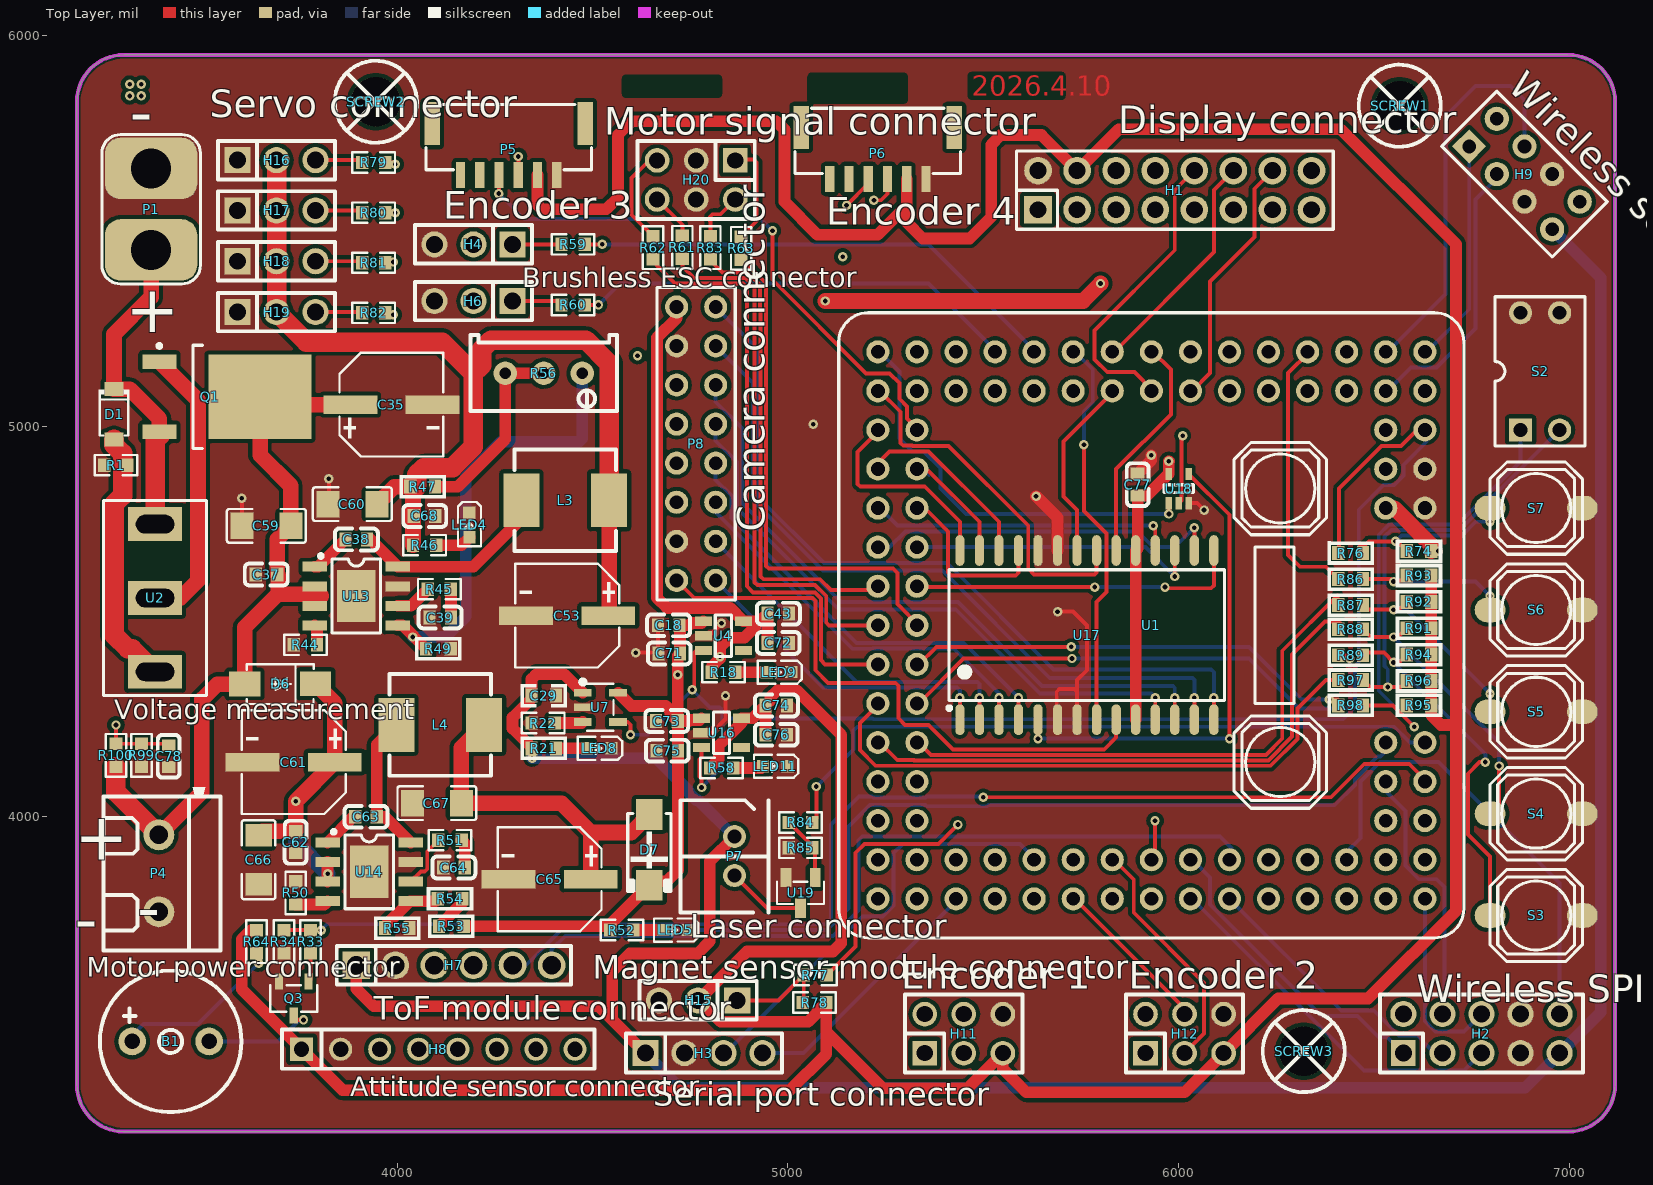
[diagram p0: Top Layer view]
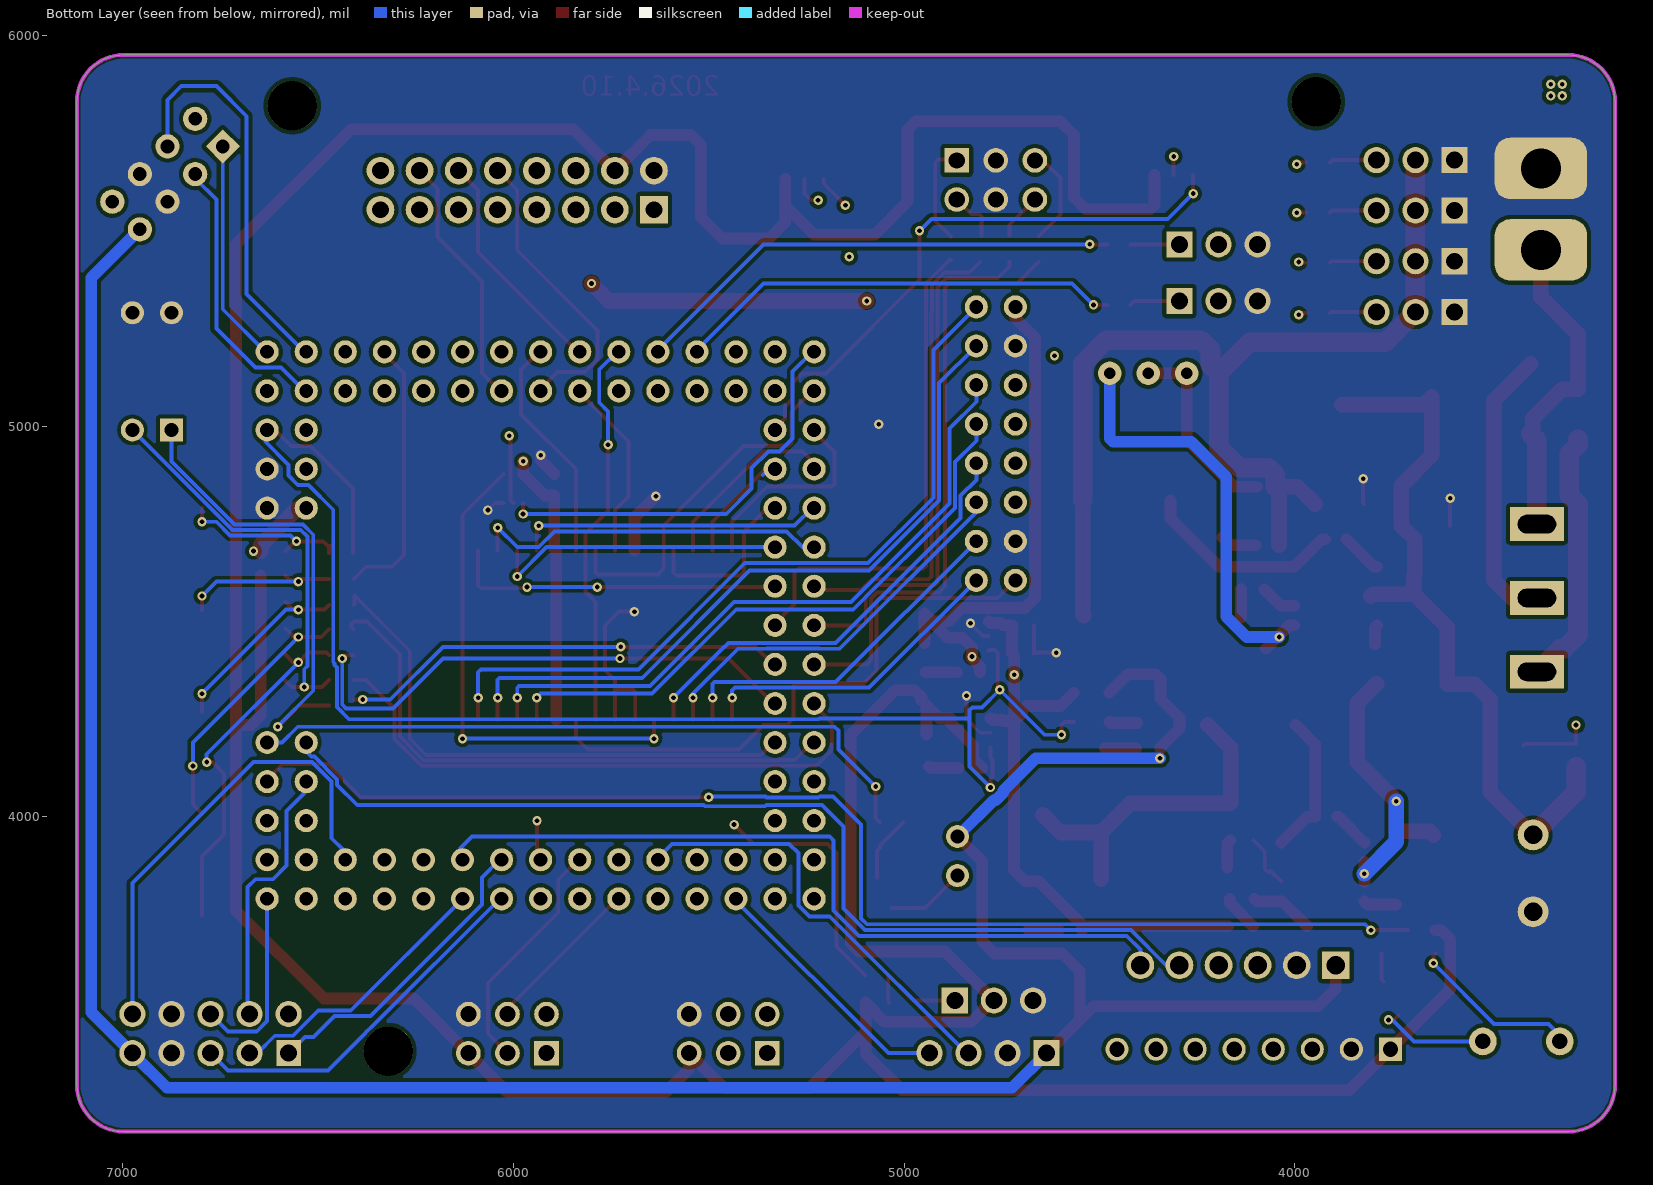
[diagram p1: Bottom Layer view, seen from below]
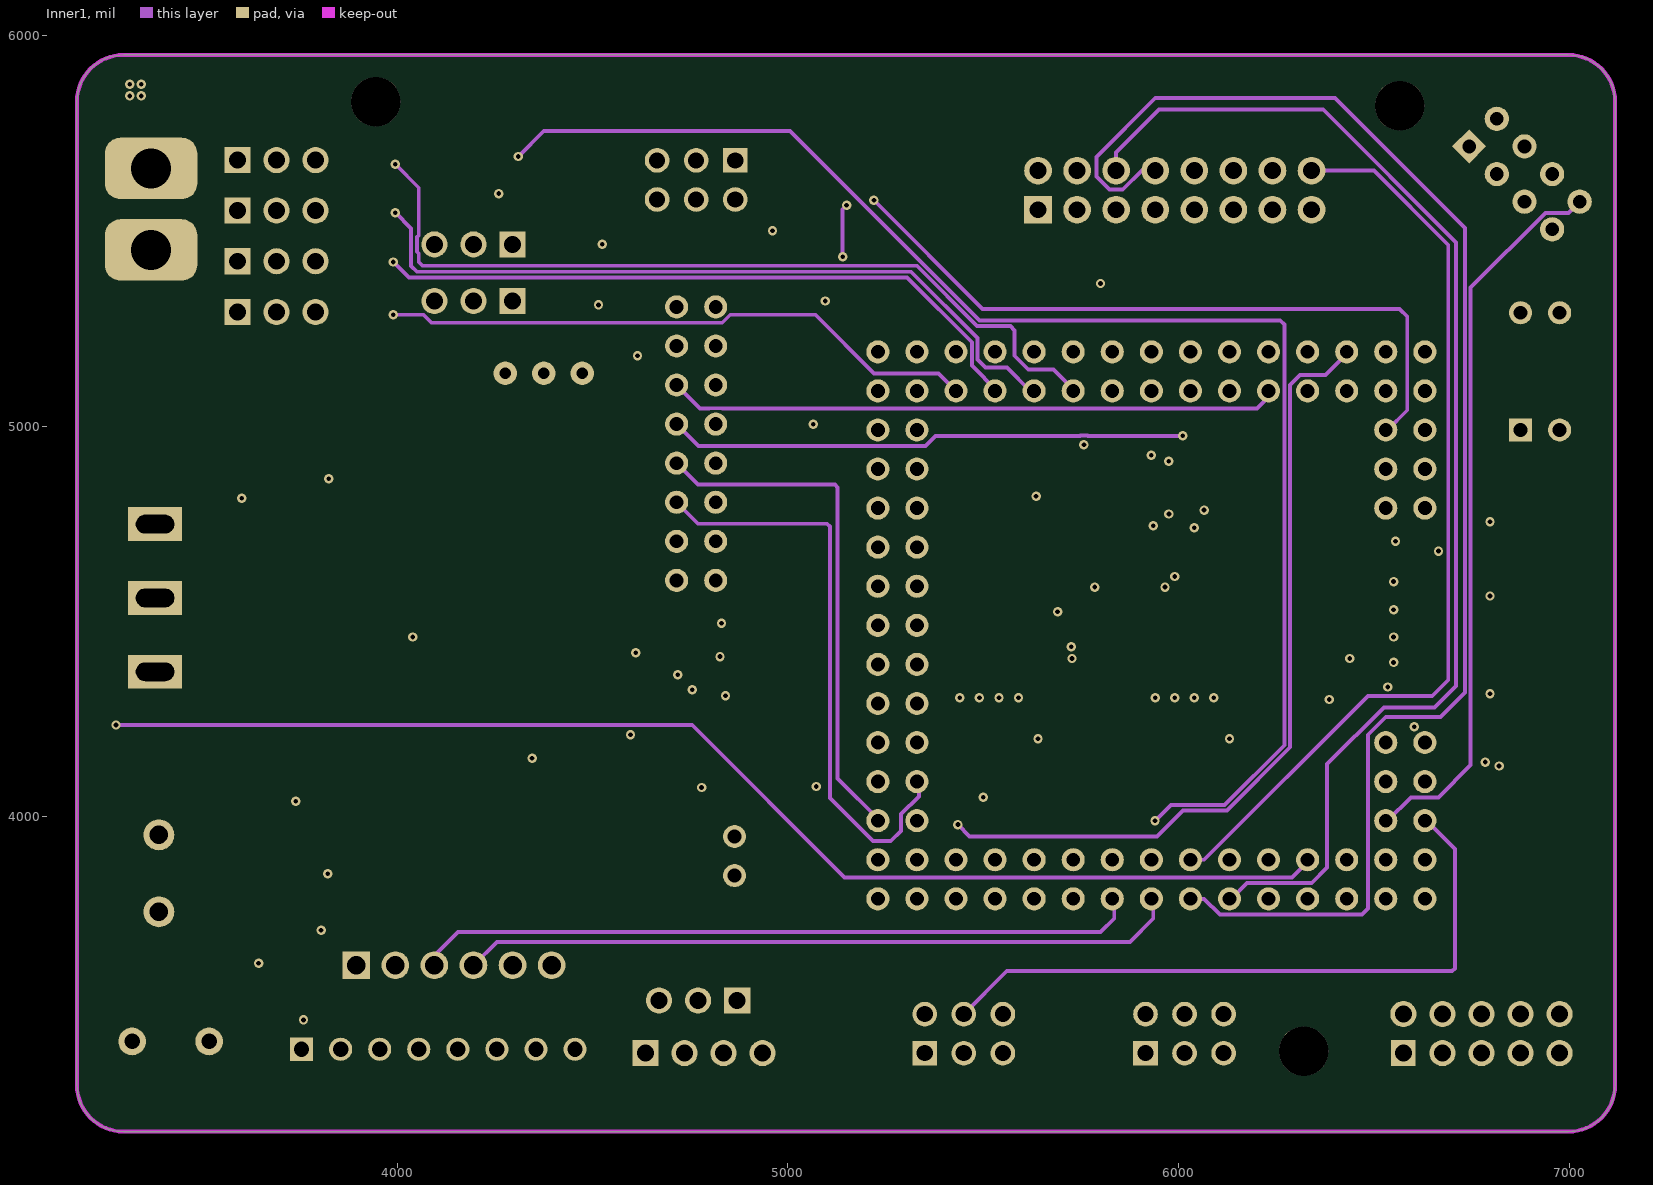
[diagram p2: Inner1]
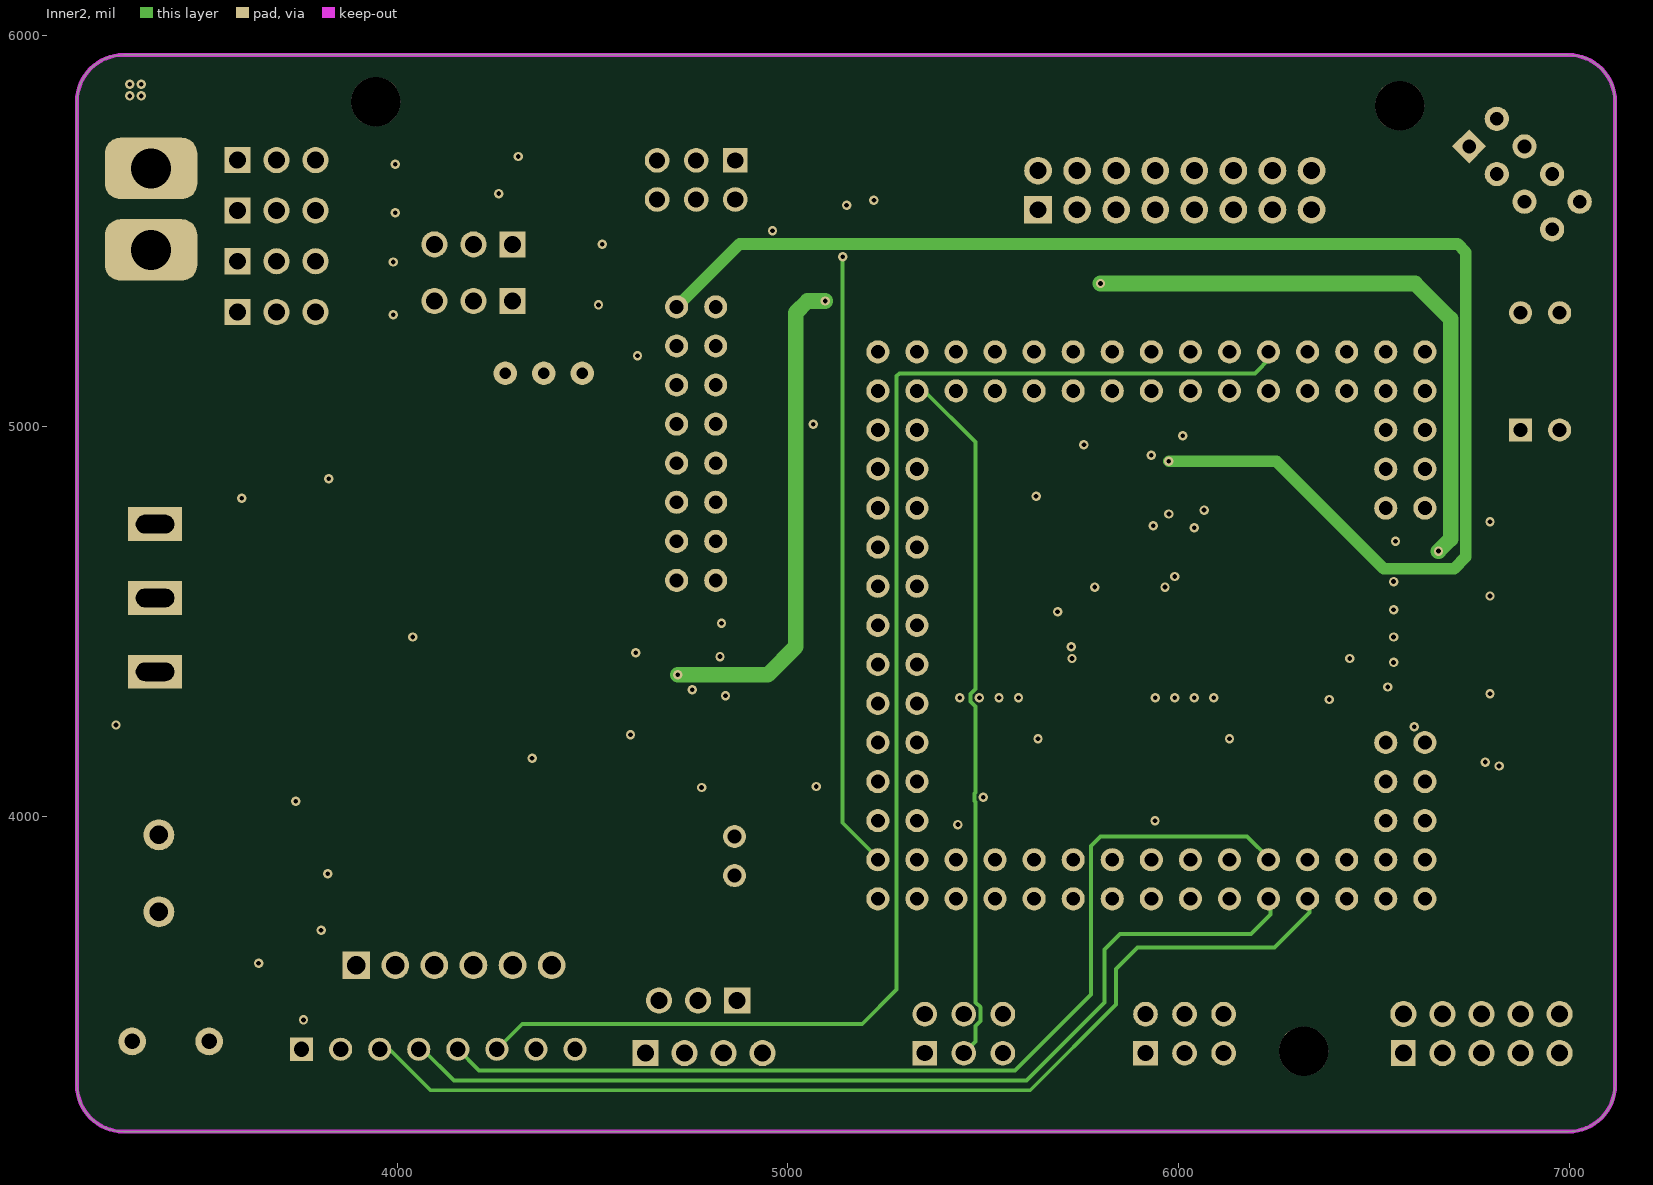
[diagram p3: Inner2]
# Altium PCB MISC49918.pcbdoc (part 1 of 2)
Units mil, origin at the board's own origin, x right, y up, seen from the top; angles counter-clockwise.
Board outline 3937.01 x 2755.91 mil, 4 copper layers (Top Layer, Inner1, Inner2, Bottom Layer), stack 62.447 mil thick; 130 components, 134 nets, 493 pads, 82 vias.

## Layer stack, top to bottom
Top Layer: signal copper 1.378
Dielectric1: surface 8.283, 7628 RC49% 8.6mil, Dk 0
Inner1: signal copper 0.598
Dielectric2: surface 41.929, 1.1mm H/HOZ Copper, Dk 0
Inner2: signal copper 0.598
Dielectric3: surface 8.283, 7628 RC49% 8.6mil, Dk 0
Bottom Layer: signal copper 1.378

## Board outline
3300,5950 ccw(c3300,5830) 3180,5830 3180,3314.09 ccw(c3300,3314.09) 3300,3194.09 6997.01,3194.09 ccw(c6997.01,3314.09) 7117.01,3314.09 7117.01,5830 ccw(c6997.01,5830) 6997.01,5950

## Design rules (kind name [scope] priority, off if disabled: settings)
BoardOutlineClearance copperThickness2oz_1 [All] p2 off: genericclearance=7.99 ignorepadtopadclearanceinfootprint=FALSE except(0: Arc-SplitContinuation Track-SplitContinuation SMDPad-SplitContinuation THPad-SplitContinuation Via-SplitContinuation Fill-SplitContinuation Region-SplitContinuation Poly-SplitContinuation Text-SplitContinuation Hole-SplitContinuation; 5.98: Arc-CutoutEdge SMDPad-CutoutEdge THPad-CutoutEdge Via-CutoutEdge Fill-CutoutEdge Region-CutoutEdge Text-CutoutEdge; 6.93: Hole-OutlineEdge Hole-CutoutEdge; 10: Poly-OutlineEdge Poly-CutoutEdge; 11.81: Arc-OutlineEdge Track-OutlineEdge SMDPad-OutlineEdge THPad-OutlineEdge Via-OutlineEdge Fill-OutlineEdge Region-OutlineEdge Text-OutlineEdge Track-CutoutEdge)
BoardOutlineClearance Plane_innerPlane_1 [All] p4 off: genericclearance=4.02 ignorepadtopadclearanceinfootprint=FALSE except(0: Arc-SplitContinuation Track-SplitContinuation SMDPad-SplitContinuation THPad-SplitContinuation Via-SplitContinuation Fill-SplitContinuation Region-SplitContinuation Poly-SplitContinuation Text-SplitContinuation Hole-SplitContinuation; 6: SMDPad-CutoutEdge THPad-CutoutEdge Via-CutoutEdge Fill-CutoutEdge Region-CutoutEdge Text-CutoutEdge; 6.93: Hole-OutlineEdge Hole-CutoutEdge; 10: Poly-OutlineEdge Poly-CutoutEdge; 11.8: Arc-OutlineEdge Track-OutlineEdge SMDPad-OutlineEdge THPad-OutlineEdge Via-OutlineEdge Fill-OutlineEdge Region-OutlineEdge Text-OutlineEdge; 11.81: Arc-CutoutEdge Track-CutoutEdge)
BoardOutlineClearance Copper_copperRegion_1 [All] p6 off: genericclearance=4.02 ignorepadtopadclearanceinfootprint=FALSE except(0: Arc-SplitContinuation Track-SplitContinuation SMDPad-SplitContinuation THPad-SplitContinuation Via-SplitContinuation Fill-SplitContinuation Region-SplitContinuation Poly-SplitContinuation Text-SplitContinuation Hole-SplitContinuation; 6: SMDPad-CutoutEdge THPad-CutoutEdge Via-CutoutEdge Fill-CutoutEdge Region-CutoutEdge Text-CutoutEdge; 6.93: Hole-OutlineEdge Hole-CutoutEdge; 10: Poly-OutlineEdge Poly-CutoutEdge; 11.8: Arc-OutlineEdge Track-OutlineEdge SMDPad-OutlineEdge THPad-OutlineEdge Via-OutlineEdge Fill-OutlineEdge Region-OutlineEdge Text-OutlineEdge; 11.81: Arc-CutoutEdge Track-CutoutEdge)
BoardOutlineClearance copperThickness1oz_1 [All] p8: genericclearance=4.02 ignorepadtopadclearanceinfootprint=FALSE except(0: Arc-SplitContinuation Track-SplitContinuation SMDPad-SplitContinuation THPad-SplitContinuation Via-SplitContinuation Fill-SplitContinuation Region-SplitContinuation Poly-SplitContinuation Text-SplitContinuation Hole-SplitContinuation; 6: SMDPad-CutoutEdge THPad-CutoutEdge Via-CutoutEdge Fill-CutoutEdge Region-CutoutEdge Text-CutoutEdge; 6.93: Hole-OutlineEdge Hole-CutoutEdge; 10: Poly-OutlineEdge Poly-CutoutEdge; 11.8: Arc-OutlineEdge Track-OutlineEdge SMDPad-OutlineEdge THPad-OutlineEdge Via-OutlineEdge Fill-OutlineEdge Region-OutlineEdge Text-OutlineEdge; 11.81: Arc-CutoutEdge Track-CutoutEdge)
Clearance copperThickness2oz [All] p1 off: gap=7.99 ignorepadtopadclearanceinfootprint=FALSE except(5.98: SMDPad-Track SMDPad-SMDPad THPad-Track SMDPad-THPad THPad-THPad Track-Via SMDPad-Via THPad-Via Via-Via Fill-Track Region-Track Fill-SMDPad Region-SMDPad Fill-THPad Region-THPad Fill-Via Region-Via Fill-Fill Fill-Region Region-Region Arc-Track Arc-SMDPad Arc-THPad Arc-Via Fill-Arc Region-Arc Arc-Arc Text-Track SMDPad-Text Text-THPad Text-Via Fill-Text Region-Text Arc-Text Text-Text; 6.93: Hole-Track Hole-SMDPad Hole-THPad Hole-Via Fill-Hole Region-Hole Hole-Arc Hole-Text; 10: Poly-Track Poly-SMDPad Poly-THPad Poly-Via Poly-Fill Poly-Region Poly-Poly Poly-Arc Poly-Text Poly-Hole)
Clearance Plane_innerPlane [All] p3 off: gap=4.02 ignorepadtopadclearanceinfootprint=FALSE except(5.98: SMDPad-Track SMDPad-SMDPad THPad-Track SMDPad-THPad THPad-THPad Track-Via SMDPad-Via THPad-Via Via-Via Fill-Track Region-Track Fill-SMDPad Region-SMDPad Fill-THPad Region-THPad Fill-Via Region-Via Fill-Fill Fill-Region Region-Region; 6: Arc-Track Arc-SMDPad Arc-THPad Arc-Via Fill-Arc Region-Arc Arc-Arc Text-Track SMDPad-Text Text-THPad Text-Via Fill-Text Region-Text Arc-Text Text-Text; 6.93: Hole-Track Hole-SMDPad Hole-THPad Hole-Via Fill-Hole Region-Hole Hole-Arc Hole-Text; 10: Poly-Track Poly-SMDPad Poly-THPad Poly-Via Poly-Fill Poly-Region Poly-Poly Poly-Arc Poly-Text Poly-Hole)
Clearance Copper_copperRegion [All] p5 off: gap=4.02 ignorepadtopadclearanceinfootprint=FALSE except(5.98: SMDPad-Track SMDPad-SMDPad THPad-Track SMDPad-THPad THPad-THPad Track-Via SMDPad-Via THPad-Via Via-Via Fill-Track Region-Track Fill-SMDPad Region-SMDPad Fill-THPad Region-THPad Fill-Via Region-Via Fill-Fill Fill-Region Region-Region; 6: Arc-Track Arc-SMDPad Arc-THPad Arc-Via Fill-Arc Region-Arc Arc-Arc Text-Track SMDPad-Text Text-THPad Text-Via Fill-Text Region-Text Arc-Text Text-Text; 6.93: Hole-Track Hole-SMDPad Hole-THPad Hole-Via Fill-Hole Region-Hole Hole-Arc Hole-Text; 10: Poly-Track Poly-SMDPad Poly-THPad Poly-Via Poly-Fill Poly-Region Poly-Poly Poly-Arc Poly-Text Poly-Hole)
Clearance copperThickness1oz [All] p7: gap=4.02 ignorepadtopadclearanceinfootprint=FALSE except(5.98: SMDPad-Track SMDPad-SMDPad THPad-Track SMDPad-THPad THPad-THPad Track-Via SMDPad-Via THPad-Via Via-Via Fill-Track Region-Track Fill-SMDPad Region-SMDPad Fill-THPad Region-THPad Fill-Via Region-Via Fill-Fill Fill-Region Region-Region; 6: Arc-Track Arc-SMDPad Arc-THPad Arc-Via Fill-Arc Region-Arc Arc-Arc Text-Track SMDPad-Text Text-THPad Text-Via Fill-Text Region-Text Arc-Text Text-Text; 6.93: Hole-Track Hole-SMDPad Hole-THPad Hole-Via Fill-Hole Region-Hole Hole-Arc Hole-Text; 10: Poly-Track Poly-SMDPad Poly-THPad Poly-Via Poly-Fill Poly-Region Poly-Poly Poly-Arc Poly-Text Poly-Hole)
DiffPairsRouting differentialPair [All] p1: maxlimit=6 minlimit=6 mostfreqgap=6 toplayer_minwidth=5 toplayer_prefwidth=10 toplayer_maxwidth=100 toplayer_mingap=6 toplayer_prefgap=6 toplayer_maxgap=6 midlayer1_minwidth=5 midlayer1_prefwidth=10 midlayer1_maxwidth=100 midlayer1_mingap=6 midlayer1_prefgap=6 midlayer1_maxgap=6 midlayer2_minwidth=5 midlayer2_prefwidth=10 midlayer2_maxwidth=100 midlayer2_mingap=6 midlayer2_prefgap=6 midlayer2_maxgap=6 bottomlayer_minwidth=5 bottomlayer_prefwidth=10 bottomlayer_maxwidth=100 bottomlayer_mingap=6 bottomlayer_prefgap=6 bottomlayer_maxgap=6 maxuncoupledlength=10
HoleToHoleClearance otherClearance [All] p1: gap=11.81 allowstackedmicrovias=TRUE
Length netLength [All] p1: minlimit=0 maxlimit=0
PasteMaskExpansion pasteMaskExpansion [All] p1: expansion=0
PlaneConnect innerPlane [All] p1: planeconnectstyle=Relief reliefexpansion=20 reliefentries=4 reliefconductorwidth=10 reliefairgap=10
PolygonConnect copperRegion [All] p1: connectstyle=Direct reliefconductorwidth=10 reliefentries=4 polygonreliefangle="90 Angle" airgapwidth=10 via.connectstyle=Relief via.reliefconductorwidth=10 via.reliefentries=4 via.polygonreliefangle="90 Angle" via.airgapwidth=10
RoutingVias viaSize [All] p1: holewidth=12.01 width=24.02 viastyle="Through Hole" minholewidth=11.81 minwidth=19.68 maxholewidth=248.03 maxwidth=393.7
SolderMaskExpansion solderMaskExpansion [IsVia] p1: expansion=-1000 istentingtop=TRUE
SolderMaskExpansion solderMaskExpansion [All] p2: expansion=2 istentingtop=FALSE
Width copperThickness2oz_2 [All] p1 off: maxlimit=100 minlimit=8 preferedwidth=10
Width copperThickness1oz_2 [All] p2: maxlimit=100 minlimit=5 preferedwidth=10

## Components (designator, comment, footprint, x,y, rotation, side; value= is the part's Value field where it differs from the comment)
B1 "3kHz" BUZ-TH_BD9.0-P5.00-D0.6-FD 3419.98,3424.99 r0 top locked
C18 "10uF" C0603 4695,4490 r0 top
C29 "100nF" CAPC1608[0603]S-N 4375,4310 r180 top
C35 "100uF" CAP-SMD_BD6.3-L6.6-W6.6-LS7.6-FD-1 3985,5055 r0 top
C37 "100nF" C0603 3665,4620 r0 top
C38 "100nF" C0603 3895,4710 r180 top
C39 "4.7nF" C0603 4110,4510 r0 top
C43 "10uF" C0603 4975,4520 r180 top locked
C53 "220uF" CAP-SMD_BD6.3-L6.6-W6.6-LS7.6-FD-1 4435,4515 r180 top
C59 "4.7uf" C1206 3664.89,4744.58 r0 top
C60 "47uf" C1206 3885,4800 r0 top
C61 "100uF" CAP-SMD_BD6.3-L6.6-W6.6-LS7.6-FD-1 3735,4140 r180 top
C62 "100nF" C0603 3740,3935 r90 top
C63 "100nF" C0603 3920,4000 r180 top
C64 "4.7nF" C0603 4145,3870 r0 top
C65 "220uF" CAP-SMD_BD6.3-L6.6-W6.6-LS7.6-FD-1 4390,3840 r180 top
C66 "4.7uf" C1206 3645,3890 r90 top
C67 "47uf" C1206 4101.34,4034.81 r0 top
C68 "100nF" C0603 4070,4770 r180 top
C71 "100nF" C0603 4695.94,4418.12 r0 top
C72 "100nF" C0603 4975,4445 r180 top locked
C73 "10uF" C0603 4690,4245 r0 top
C74 "10uF" C0603 4970,4285 r180 top locked
C75 "100nF" C0603 4690.94,4169.1 r0 top
C76 "100nF" C0603 4970,4210 r180 top locked
C77 "100nF" C0603 5895,4850 r270 top locked
C78 "100nF" C0603 3415,4155 r90 top
D1 "BZT52C16" SOD-123_L2.7-W1.6-LS3.7-RD 3275,5030 r270 top
D6 "SS54" SMA_L4.3-W2.6-LS5.0-FD 3700,4340 r0 top
D7 "SS54" SMA-L[DO-214AC] 4645,3915 r270 top
H1 "" HDR-TH_16P-P2.54-V-F-R2-C8-S2.54-1 5990,5603.7 r0 top locked
H2 "" HDR-TH_10P-P2.54-V-F-R2-C5-S2.54 6775,3445 r0 top
H3 "" HDR-TH_4P-P2.54-V-M 4785,3395 r0 top
H4 "" HDR-TH_3P-P2.54-V-M 4195.01,5465 r180 top
H6 "" HDR-TH_3P-P2.54-V-M 4195.01,5319.98 r180 top
H7 "" HDR-TH_6P-P2.54-V-M-1 4145,3620 r0 top locked
H8 "" HDR-TH_8P-P2.54-V-M 4105.01,3405.02 r0 top locked
H9 "HDR-F-2.54_2x4" HDR-F-2.54_2X4 6885,5645 r315 top locked
H11 "" HDR-TH_6P-P2.54-V-R2-C3-S2.54_A2541WV-2X3P 5450,3445 r0 top
H12 "" HDR-TH_6P-P2.54-V-R2-C3-S2.54_A2541WV-2X3P 6015,3445 r0 top
H15 "" HDR-TH_3P-P2.54-V-M 4770,3530 r180 top
H16 "" HDR-TH_3P-P2.54-V-M 3690.94,5680.58 r0 top locked
H17 "" HDR-TH_3P-P2.54-V-M 3690.94,5551.84 r0 top locked
H18 "" HDR-TH_3P-P2.54-V-M 3690.94,5421.81 r0 top
H19 "" HDR-TH_3P-P2.54-V-M 3690.94,5291.77 r0 top
H20 "" HDR-TH_6P-P2.54-V-R2-C3-S2.54_A2541WV-2X3P 4764.99,5629.91 r180 top locked
L3 "4.7uH" IND-SMD_L7.2-W6.6_GPSR07X0 4430,4810 r0 top
L4 "4.7uH" IND-SMD_L7.2-W6.6_GPSR07X0 4110,4235 r0 top
LED4 "" LED_0603 4185,4745 r270 top
LED5 "" LED_0603 4710,3710 r180 top locked
LED8 "" LED_0603 4515,4175 r180 top
LED9 "" LED_0603 4975,4370 r180 top locked
LED11 "" LED_0603 4965.65,4129.1 r180 top locked
P1 "XT60_Header" "Wired T-Header ThroughHole" 3370,5555 r180 top locked
P4 "KF301-2P terminal block" CONN-TH_XY301V-A-5.0-2P 3390,3855 r90 top
P5 "GH1.25-6P-SH new encoder board end, horizontal" ECD-GH1.25-6P-SV 4285,5725 r180 top
P6 "GH1.25-6P-SH new encoder board end, horizontal" ECD-GH1.25-6P-SV 5230.01,5715.01 r180 top locked
P7 "XH2.54-2P" XH2.54-2P-DV 4863.2,3949.46 r270 top locked
P8 "Camera Interface" HDR2X8-F-High 4715,5305 r270 top
Q1 "HY19P03" TO-252AA 3520,5075 r0 top
Q3 "S8050" SOT-23-3_L3.0-W1.7-P0.95-LS2.9-BR 3735,3535 r90 top locked
R1 "10K" R0603 3280,4900 r0 top
R18 "2.7K" R0603 4835,4370 r0 top
R21 "10K" RESC1608[0603]S-N 4375,4175 r0 top
R22 "4.7K" R0603 4373.29,4240 r0 top
R33 "4.7K" R0603 3778.02,3680.21 r270 top locked
R34 "10K" R0603 3710,3680.21 r270 top locked
R44 "200K" R0603 3765,4440 r0 top
R45 "20K" R0603 4107.57,4582.63 r0 top
R46 "10K" R0603 4070,4695 r0 top
R47 "27K" RESC1608[0603]S-N 4065,4845 r180 top
R49 "8.2K" RESC1608[0603]S-N 4105,4430 r180 top
R50 "200K" R0603 3740,3805 r270 top
R51 "20K" R0603 4135,3940 r0 top
R52 "4.7K" R0603 4575,3710 r0 top locked
R53 "51K" RESC1608[0603]S-N 4138.5,3719.81 r0 top locked
R54 "1.5K" RESC1608[0603]S-N 4135,3790 r0 top locked
R55 "10K" RESC1608[0603]S-N 4000,3715 r180 top locked
R56 "50kΩ" RES-ADJ-TH_3P-L9.5-W4.85-P2.50-BL-BS 4375,5135 r270 top
R58 "2.7K" R0603 4830,4125 r0 top
R59 "100R" R0603 4450,5465 r0 top
R60 "100R" R0603 4450,5310 r0 top
R61 "100R" R0603 4729.61,5457.49 r270 top
R62 "100R" R0603 4654.55,5456.52 r270 top
R63 "100R" R0603 4880,5455 r90 top locked
R64 "10R" R0603 3639.79,3680.21 r270 top locked
R74 "4.7K" RESC1608[0603]S-N 6615,4680 r180 top
R76 "470R" RESC1608[0603]S-N 6440,4675 r0 top
R77 "100R" R0603 5070,3595 r180 top
R78 "10K" R0603 5067.96,3524.5 r0 top
R79 "100R" R0603 3939.57,5674.65 r0 top locked
R80 "100R" R0603 3939.57,5546.32 r0 top locked
R81 "100R" R0603 3939.57,5417.98 r0 top
R82 "100R" R0603 3939.57,5289.65 r0 top
R83 "100R" R0603 4801.44,5456.52 r90 top
R84 "100R" R0603 5032.11,3985.39 r180 top locked
R85 "10K" R0603 5032.11,3920.39 r0 top locked
R86 "470R" RESC1608[0603]S-N 6440,4608.33 r0 top
R87 "470R" RESC1608[0603]S-N 6440,4541.67 r0 top
R88 "470R" RESC1608[0603]S-N 6440,4480 r0 top
R89 "470R" RESC1608[0603]S-N 6440,4413.33 r0 top
R91 "4.7K" RESC1608[0603]S-N 6615,4482.5 r180 top
R92 "4.7K" RESC1608[0603]S-N 6615,4550 r180 top
R93 "4.7K" RESC1608[0603]S-N 6615,4617.5 r180 top
R94 "4.7K" RESC1608[0603]S-N 6615,4415 r180 top
R95 "4.7K" RESC1608[0603]S-N 6615,4285 r180 top
R96 "4.7K" RESC1608[0603]S-N 6615,4347.5 r180 top
R97 "470R" RESC1608[0603]S-N 6440,4350 r0 top
R98 "470R" RESC1608[0603]S-N 6440,4285 r0 top
R99 "20K" R0603 3345.53,4157.19 r90 top
R100 "200K" R0603 3280,4157.19 r270 top
S2 "SW DIP-2" "Code SW-2-DIP-2.54" 6924.99,5139.98 r0 top locked
S3 "KEY-TS1145" TS-1199A 6915,3747.31 r180 top
S4 "KEY-TS1145" TS-1199A 6915,4007.98 r180 top
S5 "KEY-TS1145" TS-1199A 6915,4268.65 r180 top
S6 "KEY-TS1145" TS-1199A 6915,4529.33 r180 top
S7 "KEY-TS1145" TS-1199A 6915,4790 r180 top
SCREW1 "" M3螺丝 6565.67,5819.92 r0 top locked
SCREW2 "" M3螺丝 3944.99,5830.01 r0 top locked
SCREW3 "" M3螺丝 6320.01,3400.01 r0 top
U1 "STC32G144K246_CoreBoard" STC32G144K246_CoreBoard 5130,3690 r0 top
U2 "" SS12D10 3380,4560 r270 top
U4 "RT9013-33" SOT-23-5 4834.6,4463.12 r0 top
U7 "SY6280" SOT-23-5_L3.0-W1.7-P0.95-LS2.8-BL 4520,4280 r270 top
U13 "SCT2450" SOP-8E 3895,4565 r0 top
U14 "SCT2450" SOP-8E 3928.01,3859.1 r0 top
U16 "RT9013-33" SOT-23-5 4830,4215 r0 top
U17 "AL422B" SOP-28 5765,4465 r90 top
U18 "SN74LVC1G00DCKR" SOT-353 6000,4840 r90 top locked
U19 "AO3400" SOT-23-3_L2.9-W1.3-P1.90-LS2.4-BL-2 5032.11,3805.39 r180 top locked

## Footprints (in the part's own frame and the unit in brackets; to place one, negate y for a bottom-side part, rotate by r counter-clockwise, add the part's x,y. Pads: shape width x height; smd on the part's side, far side on the other; paste and mask are expansions set on the pad)
BUZ-TH_BD9.0-P5.00-D0.6-FD [mm]
  round 1.8 hole 1 copper offset 0,0: 1(-2.5,0)
  round 1.8 hole 1: 2(2.5,0)
  silkscreen extent -4.6,-4.6 4.6,4.6
C0603 [mm]
  rect 0.8x0.9 smd: 1(-0.7,0) 2(0.7,0)
  silkscreen extent -1.41,-0.71 1.39,0.72
C1206 [mm]
  rect 1.485x1.728 smd paste-100 mask+0.051: 1(-1.593,0) 2(1.593,0)
  silkscreen extent -2.56,-1.09 2.56,1.09
CAP-SMD_BD6.3-L6.6-W6.6-LS7.6-FD-1 [mm]
  rect 3.5x1.2 smd: 1(-2.67,0) 2(2.67,0)
  silkscreen extent -3.38,-3.38 3.38,3.38
CAPC1608[0603]S-N [mm]
  rect 0.8x0.9 smd: 1(-0.8,0) 2(0.8,0)
  silkscreen extent -1.5,-0.75 1.5,0.75
"Code SW-2-DIP-2.54" [mm]
  rect 1.5x1.5 hole 0.9: 1(-1.27,-3.81)
  round 1.5 hole 0.9: 2(1.27,-3.81) 3(1.27,3.81) 4(-1.27,3.81)
  silkscreen extent -2.93,-4.85 2.93,4.85
CONN-TH_XY301V-A-5.0-2P [mm]
  round 2 hole 1.2: 1(-2.5,0) 2(2.5,0)
  silkscreen extent -5,-4 5.6,3.6
ECD-GH1.25-6P-SV [mm]
  rect 1x2.8 smd: 0(-4.975,-1.25) 0(4.975,-1.25)
  rect 0.6x1.7 smd: 1(-3.125,2.1) 2(-1.875,2.1) 3(-0.625,2.1) 4(0.625,2.1) 5(1.875,2.1) 6(3.125,2.1)
  silkscreen extent -5.38,-2.5 5.38,1.75
HDR2X8-F-High [mm]
  round 1.5 hole 0.9: 1(0,0) 2(0,2.54) 3(2.54,0) 4(2.54,2.54) 5(5.08,0) 6(5.08,2.54) 7(7.62,0) 8(7.62,2.54) 9(10.16,0) 10(10.16,2.54) 11(12.7,0) 12(12.7,2.54) 13(15.24,0) 14(15.24,2.54) 15(17.78,0) 16(17.78,2.54)
  silkscreen extent -1.27,-1.27 19.05,3.81
HDR-F-2.54_2X4 [mil]
  rect 62x62 hole 35: 1(-150,-50)
  round 62 hole 35: 2(-150,50) 3(-50,-50) 4(-50,50) 5(50,-50) 6(50,50) 7(150,-50) 8(150,50)
  silkscreen extent -200,-100 200,100
HDR-TH_3P-P2.54-V-M [mm]
  rect 1.7x1.7 hole 1.1: 1(-2.54,0)
  round 1.7 hole 1.1: 2(0,0) 3(2.54,0)
  silkscreen extent -3.81,-1.25 3.81,1.25
HDR-TH_4P-P2.54-V-M [mm]
  rect 1.7x1.7 hole 1.1: 1(-3.81,0)
  round 1.7 hole 1.1: 2(-1.27,0) 3(1.27,0) 4(3.81,0)
  silkscreen extent -5.08,-1.27 5.08,1.27
HDR-TH_6P-P2.54-V-M-1 [mm]
  rect 1.8x1.8 hole 1.2: 1(-6.35,0)
  round 1.8 hole 1.2: 2(-3.81,0) 3(-1.27,0) 4(1.27,0) 5(3.81,0) 6(6.35,0)
  silkscreen extent -7.62,-1.25 7.62,1.25
HDR-TH_6P-P2.54-V-R2-C3-S2.54_A2541WV-2X3P [mm]
  rect 1.6x1.6 hole 1.05: 1(-2.54,-1.27)
  round 1.6 hole 1.05: 2(-2.54,1.27) 3(0,-1.27) 4(0,1.27) 5(2.54,-1.27) 6(2.54,1.27)
  silkscreen extent -3.81,-2.54 3.81,2.54
HDR-TH_8P-P2.54-V-M [mm]
  rect 1.5x1.5 hole 1: 1(-8.89,0)
  round 1.5 hole 1: 2(-6.35,0) 3(-3.81,0) 4(-1.27,0) 5(1.27,0) 6(3.81,0) 7(6.35,0) 8(8.89,0)
  silkscreen extent -10.16,-1.27 10.16,1.27
HDR-TH_10P-P2.54-V-F-R2-C5-S2.54 [mm]
  rect 1.575x1.7 hole 1.1: 1(-5.08,-1.27)
  round 1.7 hole 1.1: 2(-5.08,1.27) 3(-2.54,-1.27) 4(-2.54,1.27) 5(0,-1.27) 6(0,1.27) 7(2.54,-1.27) 8(2.54,1.27) 9(5.08,-1.27) 10(5.08,1.27)
  silkscreen extent -6.6,-2.54 6.6,2.54
HDR-TH_16P-P2.54-V-F-R2-C8-S2.54-1 [mm]
  rect 1.8x1.8 hole 1.1: 1(-8.89,-1.27)
  round 1.8 hole 1.1: 2(-8.89,1.27) 3(-6.35,-1.27) 4(-6.35,1.27) 5(-3.81,-1.27) 6(-3.81,1.27) 7(-1.27,-1.27) 8(-1.27,1.27) 9(1.27,-1.27) 10(1.27,1.27) 11(3.81,-1.27) 12(3.81,1.27) 13(6.35,-1.27) 14(6.35,1.27) 15(8.89,-1.27) 16(8.89,1.27)
  silkscreen extent -10.3,-2.54 10.3,2.54
IND-SMD_L7.2-W6.6_GPSR07X0 [mm]
  rect 2.35x3.5 smd: 1(-2.85,0) 2(2.85,0)
  silkscreen extent -3.3,-3.3 3.3,3.3
LED_0603 [mil]
  rect 31.5x31.5 smd paste+0 mask+2: 1(-33.5,-0.4) 2(29.5,-0.2)
  silkscreen extent -61,-30 53,30
M3螺丝 [mil]
  round 126 hole 126 paste+0 mask+4: 1(0,0)
  silkscreen extent -105,-105 105,105
R0603 [mil]
  rect 31.75x34.02 smd paste-3937.01 mask+2: 1(-29.66,0) 2(29.66,0)
  silkscreen extent -55,-26 55,26
RES-ADJ-TH_3P-L9.5-W4.85-P2.50-BL-BS [mil]
  round 60 hole 30: 1(0,98.43) 2(0,0) 3(0,-98.43)
  silkscreen extent -98,-187 96,187
RESC1608[0603]S-N [mm]
  rect 0.8x0.9 smd: 1(-0.8,0) 2(0.8,0)
  silkscreen extent -1.5,-0.75 1.5,0.75
SMA-L[DO-214AC] [mm]
  rect 2x1.75 smd: A(-2.3,0) K(2.3,0)
  silkscreen extent -2.37,-1.4 2.7,1.4
SMA_L4.3-W2.6-LS5.0-FD [mm]
  rect 2.046x1.62 smd: 1(-2.304,-0.009) 2(2.304,0.009)
  silkscreen extent -2.17,-1.32 2.19,1.29
SOD-123_L2.7-W1.6-LS3.7-RD [mm]
  rect 0.91x1.22 smd: 1(-1.635,0) 2(1.635,0)
  silkscreen extent -1.6,-1 1.38,1
SOP-8E [mm]
  rect 1.6x0.65 smd: 1(-2.7,1.905) 2(-2.7,0.635) 3(-2.7,-0.635) 4(-2.7,-1.905) 5(2.7,-1.905) 6(2.7,-0.635) 7(2.7,0.635) 8(2.7,1.905)
  rect 2.5x3.4 smd: 9(0,0)
  silkscreen extent -2.42,-2.4 1.58,2.72
SOP-28 [mm]
  oval 2x0.6 smd: 1(-5.5,8.255) 2(-5.5,6.985) 3(-5.5,5.715) 4(-5.5,4.445) 5(-5.5,3.175) 6(-5.5,1.905) 7(-5.5,0.635) 8(-5.5,-0.635) 9(-5.5,-1.905) 10(-5.5,-3.175) 11(-5.5,-4.445) 12(-5.5,-5.715) 13(-5.5,-6.985) 14(-5.5,-8.255) 15(5.5,-8.255) 16(5.5,-6.985) 17(5.5,-5.715) 18(5.5,-4.445) 19(5.5,-3.175) 20(5.5,-1.905) 21(5.5,-0.635) 22(5.5,0.635) 23(5.5,1.905) 24(5.5,3.175) 25(5.5,4.445) 26(5.5,5.715) 27(5.5,6.985) 28(5.5,8.255)
  silkscreen extent -4.87,-8.95 4.25,9.07
SOT-23-3_L2.9-W1.3-P1.90-LS2.4-BL-2 [mm]
  rect 0.7x1.25 smd: 1(-0.95,-1) 2(0.95,-1) 3(0,1)
  silkscreen extent -1.53,-0.73 1.53,0.73
SOT-23-3_L3.0-W1.7-P0.95-LS2.9-BR [mil]
  rect 40.85x20.95 smd: 1(43.36,-37.4) 2(43.36,37.4) 3(-43.36,0)
  silkscreen extent -34,-60 34,60
SOT-23-5 [mm]
  rect 1.1x0.6 smd paste+0 mask+0.102: 1(-1.3,0.95) 2(-1.3,0) 3(-1.3,-0.95) 4(1.3,-0.95) 5(1.3,0.95)
  silkscreen extent -0.53,-1.35 0.53,1.35
SOT-23-5_L3.0-W1.7-P0.95-LS2.8-BL [mm]
  rect 0.49x1.157 smd: 1(-0.95,-1.154) 2(0,-1.154) 3(0.95,-1.154)
  rect 0.49x1.175 smd: 4(0.95,1.154) 5(-0.95,1.154)
  silkscreen extent -1.8,-1.29 1.53,0.85
SOT-353 [mm]
  rect 0.8x0.4 smd: 1(-0.95,0.65) 2(-0.95,0) 3(-0.95,-0.65) 4(0.95,-0.65) 5(0.95,0.65)
  silkscreen extent -0.25,-0.95 0.25,0.95
SS12D10 [mm]
  rect 2.2x3.5 hole 1.2 slot 2.5 at 90 deg paste+0.102 mask+0.07: 1(-4.8,0) 2(0,0) 3(4.8,0)
  silkscreen extent -6.35,-3.35 6.35,3.35
STC32G144K246_CoreBoard [mm]
  round 1.5 hole 0.9: 1(38.1,27.94) 2(35.56,27.94) 3(38.1,30.48) 4(35.56,30.48) 5(38.1,33.02) 6(35.56,33.02) 7(38.1,35.56) 8(35.56,35.56) 9(38.1,38.1) 10(35.56,38.1) 11(33.02,38.1) 12(33.02,35.56) 13(30.48,38.1) 14(30.48,35.56) 15(27.94,38.1) 16(27.94,35.56) 17(25.4,38.1) 18(25.4,35.56) 19(22.86,38.1) 20(22.86,35.56) 21(20.32,38.1) 22(20.32,35.56) 23(17.78,38.1) 24(17.78,35.56) 25(15.24,38.1) 26(15.24,35.56) 27(12.7,38.1) 28(12.7,35.56) 29(10.16,38.1) 30(10.16,35.56) 31(7.62,38.1) 32(7.62,35.56) 33(5.08,38.1) 34(5.08,35.56) 35(2.54,38.1) 36(2.54,35.56) 37(2.54,33.02) 38(5.08,33.02) 39(2.54,30.48) 40(5.08,30.48) 41(2.54,27.94) 42(5.08,27.94) 43(2.54,25.4) 44(5.08,25.4) 45(2.54,22.86) 46(5.08,22.86) 47(2.54,20.32) 48(5.08,20.32) 49(2.54,17.78) 50(5.08,17.78) 51(2.54,15.24) 52(5.08,15.24) 53(2.54,12.7) 54(5.08,12.7) 55(2.54,10.16) 56(5.08,10.16) 57(2.54,7.62) 58(5.08,7.62) 59(2.54,2.54) 60(2.54,5.08) 61(5.08,2.54) 62(5.08,5.08) 63(7.62,2.54) 64(7.62,5.08) 65(10.16,2.54) 66(10.16,5.08) 67(12.7,2.54) 68(12.7,5.08) 69(15.24,2.54) 70(15.24,5.08) 71(17.78,2.54) 72(17.78,5.08) 73(20.32,2.54) 74(20.32,5.08) 75(22.86,2.54) 76(22.86,5.08) 77(25.4,2.54) 78(25.4,5.08) 79(27.94,2.54) 80(27.94,5.08) 81(30.48,2.54) 82(30.48,5.08) 83(33.02,2.54) 84(33.02,5.08) 85(38.1,2.54) 86(35.56,2.54) 87(38.1,5.08) 88(35.56,5.08) 89(38.1,7.62) 90(35.56,7.62) 91(38.1,10.16) 92(35.56,10.16) 93(38.1,12.7) 94(35.56,12.7)
  silkscreen extent 0,0 40.64,40.64
TO-252AA [mm]
  rect 6.7x5.5 smd: 1(3.275,0)
  rect 2.2x0.95 smd: 2(-3.275,2.28) 3(-3.275,-2.28)
  silkscreen extent -3.4,-3.35 -0.47,3.43
TS-1199A [mm]
  oval 2x1.6 smd: 1(-3,0) 2(3,0)
  silkscreen extent -3,-3 3,3
"Wired T-Header ThroughHole" [mm]
  rrect50% 6x4 hole 2.6: 1(0,2.65) 2(0,-2.65)
  silkscreen extent -3.2,-4.85 3.2,4.85
XH2.54-2P-DV [mm]
  round 1.5 hole 0.9: 1(0,0) 2(2.54,0)
  silkscreen extent -2.36,-3.5 4.94,2.2

## Via types
v1: diameter 24.02, hole 12, Top Layer to Bottom Layer, 82 vias

## Nets (pads, with @x,y where several pads share a name; then routed paths per layer and width w, separated by ;. In a path a pad name is that pad's centre, name@x,y a point inside that pad or via, vN(x,y) a via of type N, cw(c..) or ccw(c..) an arc to the next point about the centre after c; other vN are vias at no path point)
0.4: H3.4 U1.63 | length 663.3
  Bottom Layer w10: H3.4@4935,3395 5039.65,3395 U1.63@5434.65,3790
0.5: H3.3 U1.68 | length 1116.5
  Bottom Layer w10: H3.3@4835,3395 4840,3395 5190,3745 5242.29,3745 5270.51,3773.22 5270.51,3906.78 5294.24,3930.51 5594.13,3930.51 U1.68@5634.65,3890
1.0: C78.2 R99.2 R100.1 U1.82 | length 3419.8
  Top Layer w10: v1(3280,4235) R100.1@3280,4186.85 R99.2@3345.53,4186.85 3410.71,4186.85 C78.2@3415,4182.56
  Inner1 w10: v1(3280,4235) 4755,4235 5145,3845 6289.65,3845 U1.82@6334.65,3890
1.5: H2.6 U1.85 | length 489.7
  Bottom Layer w10: U1.85@6634.65,3790 6630,3785.35 6630,3477.14 6656.59,3450.55 6695.31,3450.55 6695.86,3450 6730,3450 H2.6@6775,3495
2.0: U1.37 U17.28 | length 537.3
  Top Layer w10: U1.37@5234.65,4990 5177.93,4933.28 5177.93,4851.9 5185,4844.83 5350.17,4844.83 5440,4755 U17.28@5440,4681.54
2.1: U1.40 U17.27 | length 317.4
  Top Layer w10: U1.40@5334.65,4890 5355,4890 5490,4755 U17.27@5490,4681.54
  Bottom Layer w10: U1.40@5335,4890 5346.5,4890 5361.5,4875
2.2: U1.39 U17.26 | length 483.5
  Top Layer w10: U1.39@5234.65,4890 5234.65,4909.65 5260,4935 5360,4935 5540,4755 U17.26@5540,4681.54
2.3: U1.42 U17.25 | length 447.6
  Top Layer w10: U1.42@5334.65,4790 5350,4790 5410,4730 5410,4625 5417.07,4617.93 5582.93,4617.93 5590,4625 U17.25@5590,4681.54
2.4: U1.41 U17.18 | length 784.2
  Top Layer w10: v1(5935,4745) 5940,4740 U17.18@5940,4681.54
  Bottom Layer w10: U1.41@5235,4790 5280,4745 v1(5935,4745)
2.5: U1.44 U17.17 | length 753
  Top Layer w10: v1(5990,4615) U17.17@5990,4681.54
  Bottom Layer w10: U1.44@5334.65,4690 5915,4690 v1(5990,4615)
2.6: U1.43 U17.16 | length 917.7
  Top Layer w10: U17.16@6040,4681.54 v1(6040,4740)
  Bottom Layer w10: U1.43@5235,4690 5260,4690 5300.51,4730.51 5894.31,4730.51 5934.82,4690 5990,4690 v1(6040,4740)
2.7: U1.46 U17.15 | length 849.8
  Top Layer w10: U1.46@5334.65,4590 5336.72,4587.93 v1(5785,4587.93) ; v1(5965,4587.93) 5967.93,4585 6082.93,4585 6090,4592.07 U17.15@6090,4681.54
  Bottom Layer w10: v1(5785,4587.93) v1(5965,4587.93)
3.2: R86.1 U1.13 | length 696.7
  Top Layer w10: U1.13@6334.65,5190 6280,5135.35 6280,4670 6310,4640 6376.84,4640 R86.1@6408.5,4608.33
3.3: P8.5 U1.16 | length 1569.8
  Inner1 w10: P8.5@4715,5105 4775,5045 4797.71,5045 4798.22,5045.51 4831.78,5045.51 4832.29,5045 6200,5045 6235,5080 U1.16@6235,5090
3.4: H8.6 U1.15 | length 3647.8
  Inner2 w10: H8.6@4255.01,3405.02 4319.99,3470 5190,3470 5277.93,3557.93 5277.93,5127.93 5285,5135 6195,5135 6235,5175 U1.15@6235,5190
3.5: H1.14 U1.20 | length 648.8
  Top Layer w10: U1.20@6034.65,5090 6080,5135.35 6080,5370 6193.58,5483.58 6193.58,5607.28 H1.14@6240,5653.7
3.7: U1.21 U17.20 | length 585.2
  Top Layer w10: U17.20@5840,4681.54 5840,4890 5980,5030 5980,5144.65 U1.21@5934.65,5190
4.0: H11.4 U1.89 | length 1713.5
  Inner1 w10: H11.4@5450,3495 5560,3605 6700,3605 6707.07,3612.07 6707.07,3917.57 U1.89@6634.65,3990
4.1: U1.35 U18.1 | length 1070.8
  Top Layer w10: U18.1@5974.41,4802.6 5975,4802.01 v1(5975,4775)
  Bottom Layer w10: U1.35@5235,5190 5285,5140 5285,4968.57 5318.57,4935 5347.29,4935 5390,4892.29 5390,4840 5455,4775 v1(5975,4775)
4.2: H11.3 U1.34 | length 1799.5
  Inner2 w10: U1.34@5334.65,5090 5348.79,5090 5480,4958.79 5480,4327.52 5467.01,4314.52 5467.01,4295.48 5480,4282.48 5480,4062.52 5477.01,4059.52 5477.01,4040.48 5480,4037.48 5480,3525.08 5492.48,3512.6 5492.48,3477.4 5480,3464.92 5480,3425 H11.3@5450,3395
4.3: U1.36 U17.21 | length 919.7
  Top Layer w10: U1.36@5234.65,5090 5287.93,5036.72 5287.93,4957.07 5295,4950 5317.35,4950 5318.34,4949.02 5410.98,4949.02 5615,4745 5615,4635 5630,4620 5785,4620 5790,4625 U17.21@5790,4681.54
4.4: P5.4 U1.38 | length 1487.2
  Top Layer w10: v1(4260,5595) 4260.39,5595.39 P5.4@4260.39,5642.32 ; v1(4960.46,5499.54) 4960.46,5374.54 5200,5135 5260,5135 5285,5110 5285,5070 5305,5050 5305,5019.65 U1.38@5334.65,4990
  Bottom Layer w10: v1(4260,5595) 4325,5530 4930,5530 v1(4960.46,5499.54)
4.6: P6.4 U1.60 | length 1808.6
  Top Layer w10: v1(5150,5565) 5205.4,5620.4 P6.4@5205.4,5632.34
  Inner1 w10: v1(5140,5433.22) 5140,5555 v1(5150,5565)
  Inner2 w10: v1(5140,5433.22) 5140,3984.65 U1.60@5234.65,3890
4.7: H2.10 U1.84 | length 1206.7
  Bottom Layer w10: U1.84@6434.65,3890 6434.65,3914.65 6465,3945 6465,4090 6515,4140 6665,4140 6975,3830 H2.10@6975,3495
5.4: H9.8 U1.90 | length 1864
  Inner1 w10: U1.90@6534.65,3990 6594.13,4049.49 6664.49,4049.49 6747.07,4132.07 6747.07,5354.31 6938.32,5545.56 6997.69,5545.56 H9.8@7026.42,5574.29
6.0: H12.4 U1.69 | length 411.1
  Top Layer w10: U1.69@5734.65,3790 6015,3509.65 H12.4@6015,3495
6.1: H7.3 U1.71 | length 1854.4
  Inner1 w10: H7.3@4095,3620 4095,3645 4155,3705 5800,3705 5835,3740 U1.71@5835,3790
6.2: H12.3 U1.72 | length 611.1
  Top Layer w10: U1.72@5834.65,3890 5885,3839.65 5885,3755 6065,3575 6065,3445 H12.3@6015,3395
6.3: H7.4 U1.73 | length 1839.7
  Inner1 w10: H7.4@4195,3620 4255,3680 5875,3680 5935,3740 U1.73@5935,3790
6.4: H2.4 U1.92 | length 683.6
  Bottom Layer w10: U1.92@6534.65,4090 6534.65,4060.35 6580,4015 6580,3875 6615,3840 6660,3840 6680,3820 6680,3500 H2.4@6675,3495
6.5: R33.1 R34.1 U1.91 | length 3264.2
  Top Layer w10: R34.1@3710,3709.87 R33.1@3778.02,3709.87 v1(3805,3709.87) ; v1(5500,4050) 6390,4050 6475,4135 6590,4135 U1.91@6635,4090
  Bottom Layer w10: v1(3805,3709.87) 3820.13,3725 5095,3725 5110,3740 5110,3980 5182.07,4052.07 5215.64,4052.07 5218.22,4049.49 5351.78,4049.49 5354.36,4052.07 5497.93,4052.07 v1(5500,4050)
6.6: H7.5 U1.94 | length 2620.5
  Bottom Layer w10: H7.5@4295,3620 4329.36,3620 4419.36,3710 5099.82,3710 5155,3765.18 5155,3975 5210,4030 5217.71,4030 5218.22,4030.51 5351.78,4030.51 5355.28,4027.01 5509.52,4027.01 5512.52,4030 6399.32,4030 6450.98,4081.66 6450.98,4095.81 6509.19,4154.02 6516.52,4154.02 6535,4172.5 U1.94@6535,4190
6.7: R84.1 U1.93 | length 1767.3
  Top Layer w10: R84.1@5061.77,3985.39 5072.5,3996.11 v1(5072.5,4077.5)
  Bottom Layer w10: v1(5072.5,4077.5) 5167.5,4172.5 5167.5,4220.51 5177.5,4230.51 6551.78,4230.51 6592.29,4190 U1.93@6635,4190
7.0: H1.10 U1.22 | length 772.1
  Top Layer w10: U1.22@5934.65,5090 5886.72,5137.93 5817.07,5137.93 5785,5170 5785,5245 5990,5450 5990,5603.7 H1.10@6040,5653.7
7.1: H1.12 U1.23 | length 590.4
  Top Layer w10: U1.23@5834.65,5190 5835,5190 6090,5445 6090,5603.7 H1.12@6140,5653.7
7.2: U1.24 U17.22 | length 476.7
  Top Layer w10: U17.22@5740,4681.54 5740,4785 5705,4820 5705,4960.35 U1.24@5834.65,5090